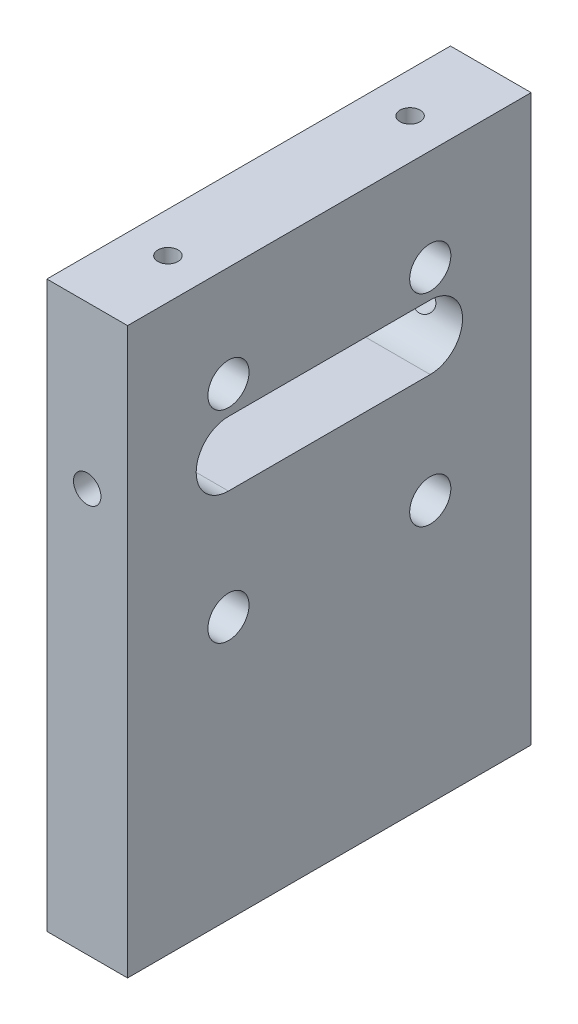
SolidWorks part; units mm, degrees
ref_plane "前视基准面" through (0, 0, 0) normal (0, 0, 1) x (1, 0, 0)
ref_plane "上视基准面" through (0, 0, 0) normal (0, 1, 0) x (1, 0, 0)
ref_plane "右视基准面" through (0, 0, 0) normal (1, 0, 0) x (0, 0, -1)
sketch "草图1" plane through (0, 0, 0) normal (1, 0, 0) x (0, 0, -1)
  line L1 (-50, 70) -> (50, 70)
  line L2 (-50, 70) -> (-50, -70)
  line L3 (-50, -70) -> (50, -70)
  line L4 (50, 70) -> (50, -70)
  line L5 (-50, 70) -> (50, -70) construction
  line L6 (-50, -70) -> (50, 70) construction
  point P0 (0, 0)
  dimension "D1" = 100
  dimension "D2" = 140
extrude "凸台-拉伸1" add sketch "草图1" along normal blind 20
hole_wizard "M6 螺纹孔1" positions "草图2" profile "草图3" tap size "M6" standard "GB"
sketch "草图2" plane through (0, -70, 0) normal (0, -1, 0) x (-1, 0, 0)
  line L0 (-10, -50) -> (-10, 47.319) construction
  line L1 (-20, -50) -> (0, -50) construction
  line L3 (0, 0) -> (-16.4512, 0) construction
  point P0 (-10, 30)
  point P2 (-10, -30)
  dimension "D1" = 60
sketch "草图3" plane through (10, -70, -30) normal (1, 0, 0) x (0, 0, -1)
  line L0 (0, 0) -> (0, 16.5022)
  line L1 (0, 16.5022) -> (2.5, 15)
  line L2 (2.5, 15) -> (2.5, 0)
  line L5 (2.5, 0) -> (0, 0)
  line L10 (0, 16.5022) -> (-2.5, 15) construction
  line L11 (0, -6.35) -> (0, 107.95) construction
  dimension "螺纹孔钻头直径" = 5
  dimension "螺纹孔钻头深度" = 15
  dimension "导头角度" = 118
cosmetic thread "孔螺蚊线1" parameters "D1"=12, "D2"=6
cosmetic thread "孔螺蚊线2" parameters "D1"=12, "D2"=6
sketch "草图4" plane through (0, 0, 0) normal (-1, 0, 0) x (0, 0, 1)
  line L0 (-25, 30) -> (25, 30) construction
  line L1 (-25, 38) -> (25, 38)
  line L2 (-25, 22) -> (25, 22)
  line L3 (0, -70) -> (0, 43.5925) construction
  line L4 (50, -70) -> (-50, -70) construction
  arc A0 (-25, 38) -> (-25, 22) centre (-25, 30) ccw
  arc A1 (25, 22) -> (25, 38) centre (25, 30) ccw
  point P2 (0, 30)
  dimension "D1" = 16
  dimension "D2" = 50
  dimension "D3" = 100
extrude "切除-拉伸1" cut sketch "草图4" against normal through all
hole_wizard "M8 螺纹孔1" positions "草图5" profile "草图6" tap size "M8" standard "GB" end condition through all
sketch "草图5" plane through (0, 0, 50) normal (0, 0, 1) x (1, 0, 0)
  line L0 (0, 38) -> (0, 22) construction
  line L2 (0, 30) -> (26.2444, 30) construction
  line L4 (10, 70) -> (10, 5.2092) construction
  line L5 (20, 70) -> (0, 70) construction
  point P0 (10, 30)
sketch "草图6" plane through (10, 30, 50) normal (1, 0, 0) x (0, -1, 0)
  line L0 (0, 0) -> (0, 100)
  line L1 (0, 100) -> (3.4, 100)
  line L2 (3.4, 100) -> (3.4, 0)
  line L5 (3.4, 0) -> (0, 0)
  line L11 (0, -6.35) -> (0, 107.95) construction
  dimension "通孔螺纹孔钻头直径" = 6.8
  dimension "通孔螺纹孔钻头深度" = 100
cosmetic thread "孔螺蚊线3"
hole_wizard "M12 螺纹孔1" positions "草图7" profile "草图8" tap size "M12" standard "GB" end condition through all
sketch "草图7" plane through (0, 0, 0) normal (-1, 0, 0) x (0, 0, 1)
  line L0 (0, -70) -> (0, 87.4043) construction
  line L1 (50, -70) -> (-50, -70) construction
  point P0 (-25, 45)
  point P2 (25, 45)
  point P4 (-25, -5)
  point P6 (25, -5)
  dimension "D3" = 50
  dimension "D1" = 50
  dimension "D2" = 65
sketch "草图8" plane through (0, 45, -25) normal (0, 1, 0) x (0, 0, 1)
  line L0 (0, 0) -> (0, 20)
  line L1 (0, 20) -> (5.1, 20)
  line L2 (5.1, 20) -> (5.1, 0.925)
  line L3 (5.1, 0.925) -> (6.025, 0)
  line L5 (6.025, 0) -> (0, 0)
  line L6 (-5.1, 0.925) -> (-6.025, 0) construction
  line L11 (0, -6.35) -> (0, 107.95) construction
  dimension "通孔螺纹孔钻头直径" = 10.2
  dimension "通孔螺纹孔钻头深度" = 20
  dimension "近端锥形沉头孔直径" = 12.05
  dimension "近端锥形沉头孔角度" = 90
cosmetic thread "孔螺蚊线4"
cosmetic thread "孔螺蚊线5"
cosmetic thread "孔螺蚊线6"
cosmetic thread "孔螺蚊线7"
hole_wizard "M6 螺纹孔2" positions "草图9" profile "草图10" tap size "M6" standard "GB"
sketch "草图9" plane through (0, 70, 0) normal (0, 1, 0) x (1, 0, 0)
  line L0 (10, -50) -> (10, 57.0642) construction
  line L1 (20, -50) -> (0, -50) construction
  line L3 (0, 0) -> (32.5571, 0) construction
  point P0 (10, 30)
  point P2 (10, -30)
  dimension "D1" = 60
sketch "草图10" plane through (10, 70, -30) normal (1, 0, 0) x (0, 0, 1)
  line L0 (0, 0) -> (0, 16.5022)
  line L1 (0, 16.5022) -> (2.5, 15)
  line L2 (2.5, 15) -> (2.5, 0)
  line L5 (2.5, 0) -> (0, 0)
  line L10 (0, 16.5022) -> (-2.5, 15) construction
  line L11 (0, -6.35) -> (0, 107.95) construction
  dimension "螺纹孔钻头直径" = 5
  dimension "螺纹孔钻头深度" = 15
  dimension "导头角度" = 118
cosmetic thread "孔螺蚊线8"
cosmetic thread "孔螺蚊线9"
